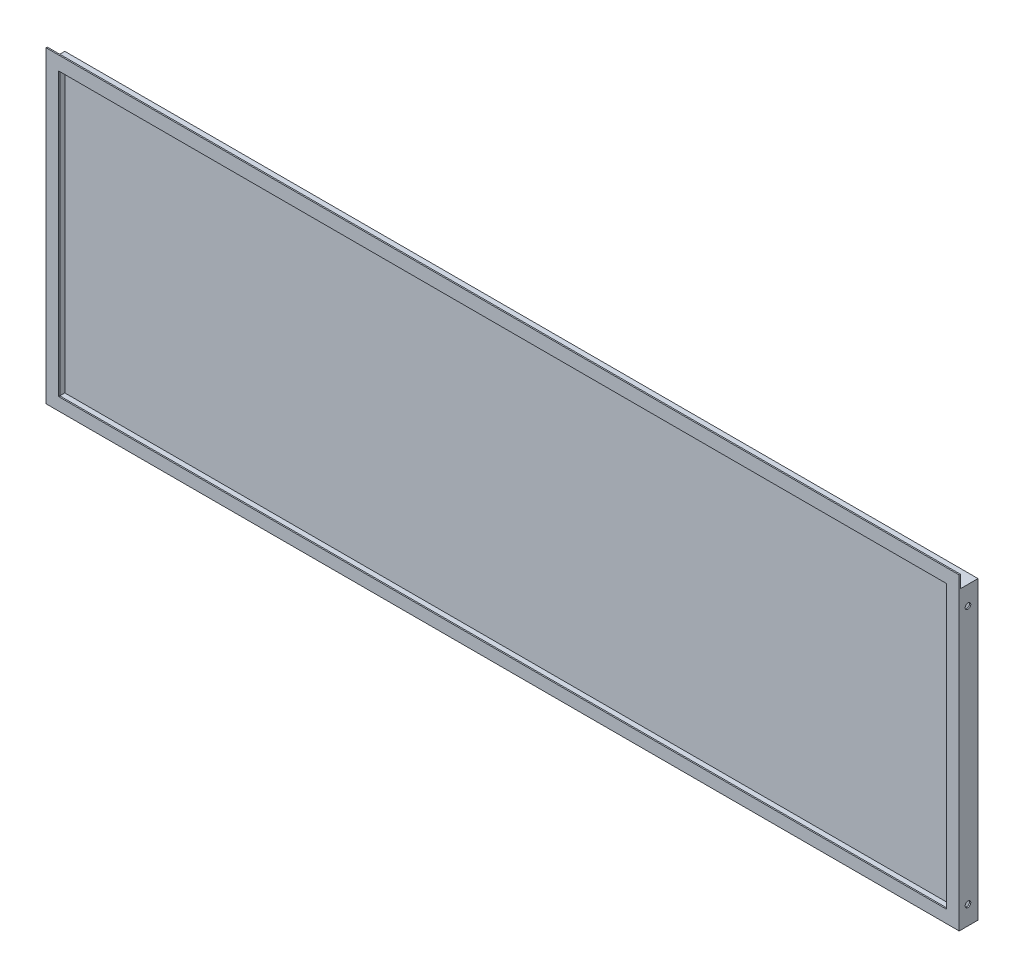
from build123d import *

# Parameters (mm, degrees)
SKETCH_1_W               = 1457
SKETCH_1_H               = 472
EXTRUDE_1_DEPTH          = 30
SHELL_1_T                = -2
SKETCH_2_W               = 1457
SKETCH_2_H               = 492
SKETCH_2_W_2             = 1417
SKETCH_2_H_2             = 450
EXTRUDE_2_DEPTH          = 2
CUT_EXTRUDE_1_DEPTH      = 1501
CUT_EXTRUDE_1_DEPTH_BACK = 10
SKETCH_3_R               = 4.5
SKETCH_6_R               = 4.5
CUT_EXTRUDE_2_DEPTH      = 10


with BuildPart() as part:
    # 草图1 → 凸台-拉伸1 (new body)
    with BuildSketch(Plane.XY):
        with Locations((728.5, 236)):
            Rectangle(SKETCH_1_W, SKETCH_1_H)
    extrude(amount=EXTRUDE_1_DEPTH)

    # 抽壳1
    shell_1_openings = [part.faces().sort_by_distance(p)[0] for p in [
        (728.5, 236, 30),
    ]]
    offset(amount=SHELL_1_T, openings=shell_1_openings, kind=Kind.INTERSECTION)

    # 草图2 → 凸台-拉伸2 (add)
    with BuildSketch(Plane.XY.offset(30)):
        with Locations((728.5, 246)):
            Rectangle(SKETCH_2_W, SKETCH_2_H)
        with Locations((728.5, 245)):
            Rectangle(SKETCH_2_W_2, SKETCH_2_H_2, mode=Mode.SUBTRACT)
    extrude(amount=-EXTRUDE_2_DEPTH)

    # 草图3 → 切除-拉伸1 (cut, two sides: drawn at the far end of the back side and taken through both)
    with BuildSketch(Plane(origin=(2, 0, 0), x_dir=(0, 0, -1), z_dir=(1, 0, 0)).offset(-CUT_EXTRUDE_1_DEPTH_BACK)):
        with Locations(Location((-16, 442, 0), (0, 0, 180))):
            Circle(SKETCH_3_R)
        with Locations(Location((-16, 30, 0), (0, 0, 180))):
            Circle(SKETCH_3_R)
    extrude(amount=CUT_EXTRUDE_1_DEPTH + CUT_EXTRUDE_1_DEPTH_BACK, mode=Mode.SUBTRACT)

    # 草图6 → 切除-拉伸2 (cut)
    with BuildSketch(Plane(origin=(0, 2, 0), x_dir=(1, 0, 0), z_dir=(0, 1, 0))):
        with Locations(Location((30, -16, 0), (0, 0, 270))):
            Circle(SKETCH_6_R)
        with Locations(Location((450, -16, 0), (0, 0, 270))):
            Circle(SKETCH_6_R)
        with Locations(Location((1427, -16, 0), (0, 0, 270))):
            Circle(SKETCH_6_R)
        with Locations(Location((968.5, -16, 0), (0, 0, 270))):
            Circle(SKETCH_6_R)
        with Locations(Location((510, -16, 0), (0, 0, 270))):
            Circle(SKETCH_6_R)
        with Locations(Location((78, -16, 0), (0, 0, 270))):
            Circle(SKETCH_6_R)
        with Locations(Location((178, -16, 0), (0, 0, 270))):
            Circle(SKETCH_6_R)
    extrude(amount=-CUT_EXTRUDE_2_DEPTH, mode=Mode.SUBTRACT)


solid = part.part
